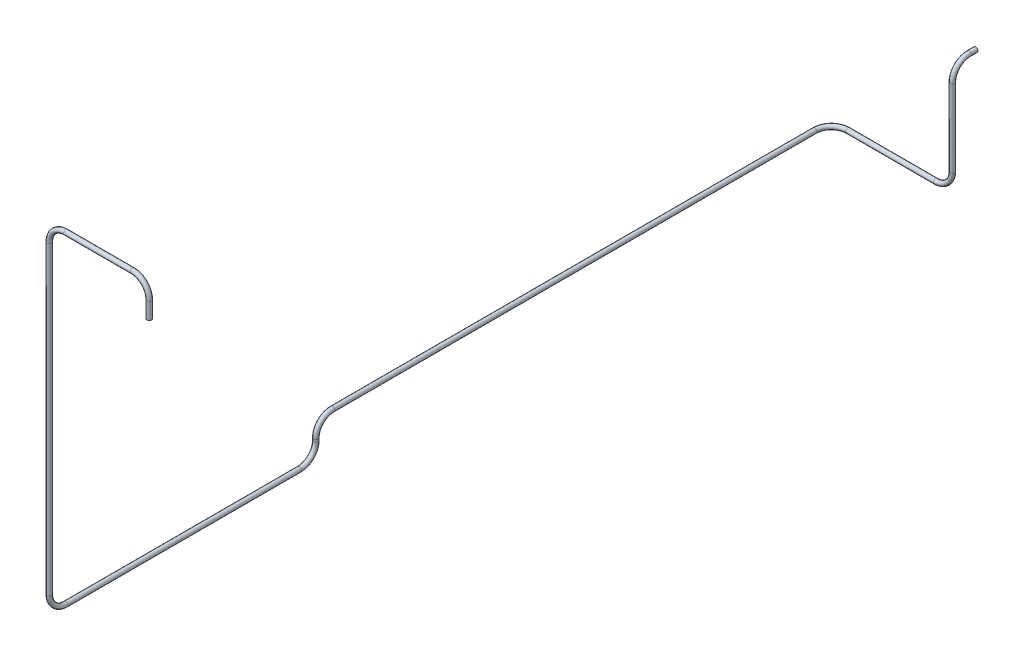
SolidWorks part; units mm, degrees
ref_plane "Front Plane" through (0, 0, 0) normal (0, 0, 1) x (1, 0, 0)
ref_plane "Top Plane" through (0, 0, 0) normal (0, 1, 0) x (1, 0, 0)
ref_plane "Right Plane" through (0, 0, 0) normal (1, 0, 0) x (0, 0, -1)
sketch "Sketch 1" plane through (0, 0, 0) normal (0, 0, 1) x (1, 0, 0)
  line L0 (0, 208.6331) -> (0, -141.7266) construction
  line L1 (-142.446, 0) -> (127.3381, 0) construction
  line L2 (150, 0) -> (150, 50)
  line L3 (100, 100) -> (-100, 100)
  line L4 (-150, 50) -> (-150, -816.5)
  arc A0 (-100, 100) -> (-150, 50) centre (-100, 50) ccw
  arc A1 (150, 50) -> (100, 100) centre (100, 50) ccw
  point P13 (-150, 100)
  point P16 (150, 100)
  dimension "D3" = 50
  dimension "D1" = 100
  dimension "D2" = 300
  dimension "D4" = 816.5
sketch "Sketch 2" plane through (0, 0, 0) normal (0, 1, 0) x (1, 0, 0)
  circle A0 centre (150, 0) radius 4
  circle A1 centre (150, 0) radius 7
  dimension "D1" = 8
  dimension "D2" = 3
sweep "Sweep 1" add profiles "Sketch 2" path "Sketch 1"
ref_plane "Plane 1" through (-150, 0, 0) normal (1, 0, 0) x (0, 0, -1)
sketch "Sketch 3" plane through (-150, 0, 0) normal (1, 0, 0) x (0, 0, -1)
  line L0 (0, -816.5) -> (0, -866.5)
  line L1 (-7, -816.5) -> (7, -816.5) construction
  line L2 (50, -916.5) -> (750, -916.5)
  line L3 (800, -866.5) -> (800, -859.5)
  line L4 (850, -809.5) -> (2247.5, -809.5)
  arc A0 (800, -859.5) -> (850, -809.5) centre (850, -859.5) cw
  arc A1 (750, -916.5) -> (800, -866.5) centre (750, -866.5) ccw
  arc A2 (0, -866.5) -> (50, -916.5) centre (50, -866.5) ccw
  point P10 (800, -809.5)
  point P13 (800, -916.5)
  point P16 (0, -916.5)
  dimension "D3" = 50
  dimension "D1" = 100
  dimension "D2" = 107
  dimension "D4" = 850
  dimension "D5" = 1397.5
sketch "Sketch 4" plane through (0, -816.5, 0) normal (0, -1, 0) x (1, 0, 0)
  circle A0 centre (-150, 0) radius 4 construction
  circle A1 centre (-150, 0) radius 7
  circle A2 centre (-150, 0) radius 7
  circle A3 centre (-150, 0) radius 4
  dimension "D1" = 0
sweep "Sweep 2" add profiles "Sketch 4" path "Sketch 3"
ref_plane "Plane 2" through (0, -809.5, 0) normal (0, 1, 0) x (1, 0, 0)
sketch "Sketch 5" plane through (0, -809.5, 0) normal (0, 1, 0) x (1, 0, 0)
  line L0 (-150, 2247.5) -> (-150, 2297.5)
  line L1 (-143, 2247.5) -> (-157, 2247.5) construction
  line L2 (-100, 2347.5) -> (113.2, 2347.5)
  arc A0 (-150, 2297.5) -> (-100, 2347.5) centre (-100, 2297.5) cw
  point P7 (-150, 2347.5)
  dimension "D2" = 50
  dimension "D1" = 100
  dimension "D3" = 213.2
sketch "Sketch 6" plane through (0, 0, -2247.5) normal (0, 0, -1) x (-1, 0, 0)
  circle A0 centre (150, -809.5) radius 4 construction
  circle A1 centre (150, -809.5) radius 7
  circle A2 centre (150, -809.5) radius 7
  circle A3 centre (150, -809.5) radius 4
  dimension "D1" = 0
sweep "Sweep 3" add profiles "Sketch 6" path "Sketch 5"
ref_plane "Plane 3" through (0, 0, -2347.5) normal (0, 0, 1) x (1, 0, 0)
sketch "Sketch 7" plane through (0, 0, -2347.5) normal (0, 0, 1) x (1, 0, 0)
  line L0 (113.2, -809.5) -> (163.2, -809.5)
  line L1 (-100, -809.5) -> (113.2, -809.5) construction
  line L2 (213.2, -759.5) -> (213.2, -577.5)
  arc A0 (163.2, -809.5) -> (213.2, -759.5) centre (163.2, -759.5) ccw
  point P7 (213.2, -809.5)
  dimension "D3" = 50
  dimension "D1" = 232
  dimension "D2" = 100
sketch "Sketch 8" plane through (113.2, 0, 0) normal (1, 0, 0) x (0, 0, -1)
  circle A0 centre (2347.5, -809.5) radius 4 construction
  circle A1 centre (2347.5, -809.5) radius 7
  circle A2 centre (2347.5, -809.5) radius 7
  circle A3 centre (2347.5, -809.5) radius 4
  dimension "D1" = 0
sweep "Sweep 4" add profiles "Sketch 8" path "Sketch 7"
ref_plane "Plane 4" through (213.2, 0, 0) normal (1, 0, 0) x (0, 0, -1)
sketch "Sketch 9" plane through (213.2, 0, 0) normal (1, 0, 0) x (0, 0, -1)
  line L0 (2347.5, -577.5) -> (2347.5, -527.5)
  line L1 (2354.5, -577.5) -> (2340.5, -577.5) construction
  line L2 (2397.5, -477.5) -> (2417.5, -477.5)
  arc A0 (2347.5, -527.5) -> (2397.5, -477.5) centre (2397.5, -527.5) cw
  point P7 (2347.5, -477.5)
  dimension "D2" = 50
  dimension "D1" = 100
  dimension "D3" = 20
sketch "Sketch 10" plane through (0, -577.5, 0) normal (0, 1, 0) x (1, 0, 0)
  circle A0 centre (213.2, 2347.5) radius 4 construction
  circle A1 centre (213.2, 2347.5) radius 7
  circle A2 centre (213.2, 2347.5) radius 7
  circle A3 centre (213.2, 2347.5) radius 4
  dimension "D1" = 0
sweep "Sweep 5" add profiles "Sketch 10" path "Sketch 9"
